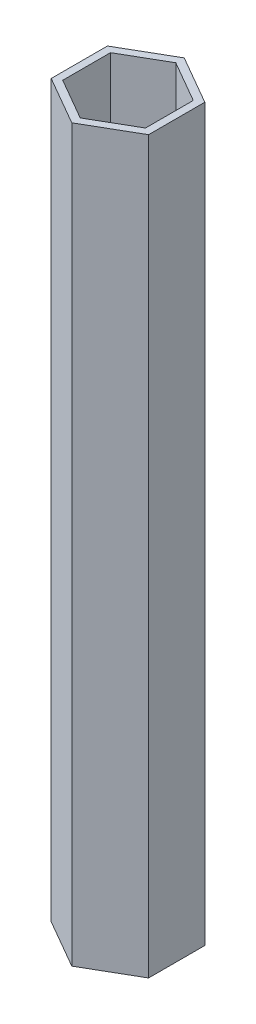
from build123d import *

# Parameters (mm, degrees)
BOSS_EXTRUDE1_DEPTH = 300


with BuildPart() as part:
    # Sketch1 → Boss-Extrude1 (new body)
    with BuildSketch(Plane(origin=(0, 0, 0), x_dir=(1, 0, 0), z_dir=(0, 1, 0))):
        Polygon((0, 23.094010768), (-20, 11.547005384), (-20, -11.547005384), (0, -23.094010768), (20, -11.547005384), (20, 11.547005384), align=None)
        Polygon((-17, 9.814954576), (-17, -9.814954576), (0, -19.629909152), (17, -9.814954576), (17, 9.814954576), (0, 19.629909152), align=None, mode=Mode.SUBTRACT)
    extrude(amount=BOSS_EXTRUDE1_DEPTH)


solid = part.part
